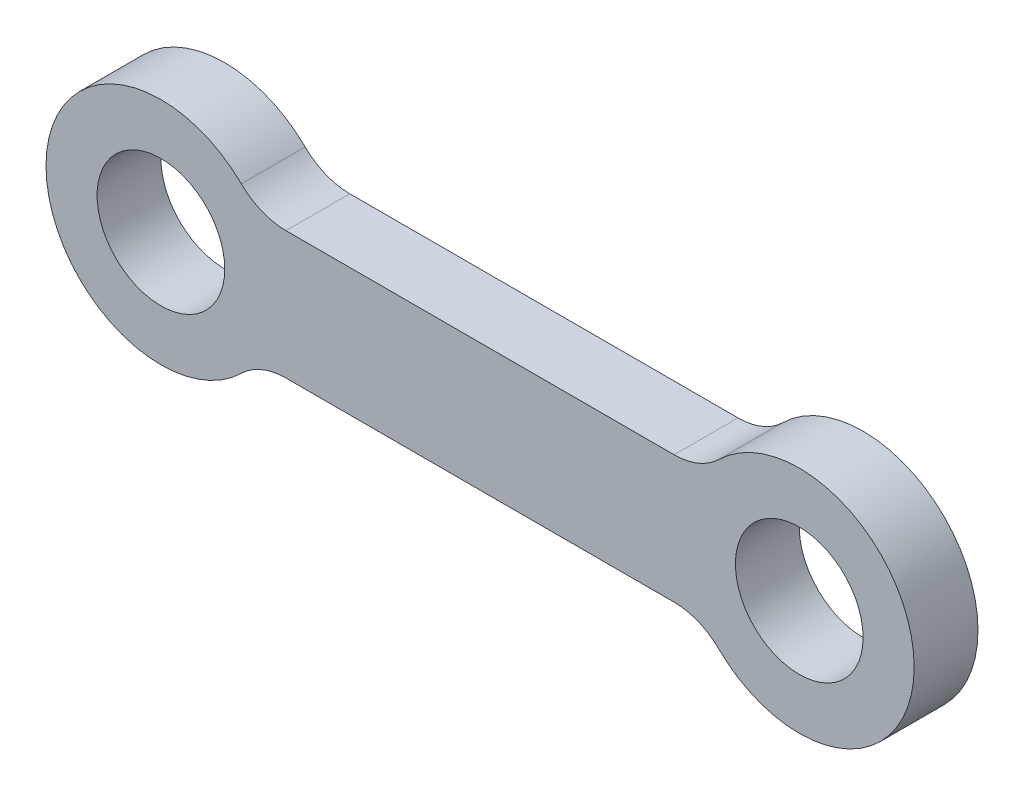
SolidWorks part; units mm, degrees
ref_plane "Front Plane" through (0, 0, 0) normal (0, 0, 1) x (1, 0, 0)
ref_plane "Top Plane" through (0, 0, 0) normal (0, 1, 0) x (1, 0, 0)
ref_plane "Right Plane" through (0, 0, 0) normal (1, 0, 0) x (0, 0, -1)
sketch "Sketch1" plane through (0, 0, 0) normal (0, 0, 1) x (1, 0, 0)
  line L0 (9.798, 5) -> (40.202, 5)
  line L1 (9.798, -5) -> (40.202, -5)
  circle A0 centre (0, 0) radius 5
  arc A1 (6.2987, 6.4286) -> (6.2987, -6.4286) centre (0, 0) ccw
  circle A2 centre (50, 0) radius 5
  arc A3 (43.7013, -6.4286) -> (43.7013, 6.4286) centre (50, 0) ccw
  arc A4 (40.202, 5) -> (43.7013, 6.4286) centre (40.202, 10) ccw
  arc A5 (40.202, -5) -> (43.7013, -6.4286) centre (40.202, -10) cw
  arc A6 (9.798, -5) -> (6.2987, -6.4286) centre (9.798, -10) ccw
  arc A7 (9.798, 5) -> (6.2987, 6.4286) centre (9.798, 10) cw
  dimension "D1" = 10
  dimension "D3" = 18
  dimension "D4" = 5
  dimension "D2" = 50
extrude "Boss-Extrude1" add sketch "Sketch1" along normal blind 5
